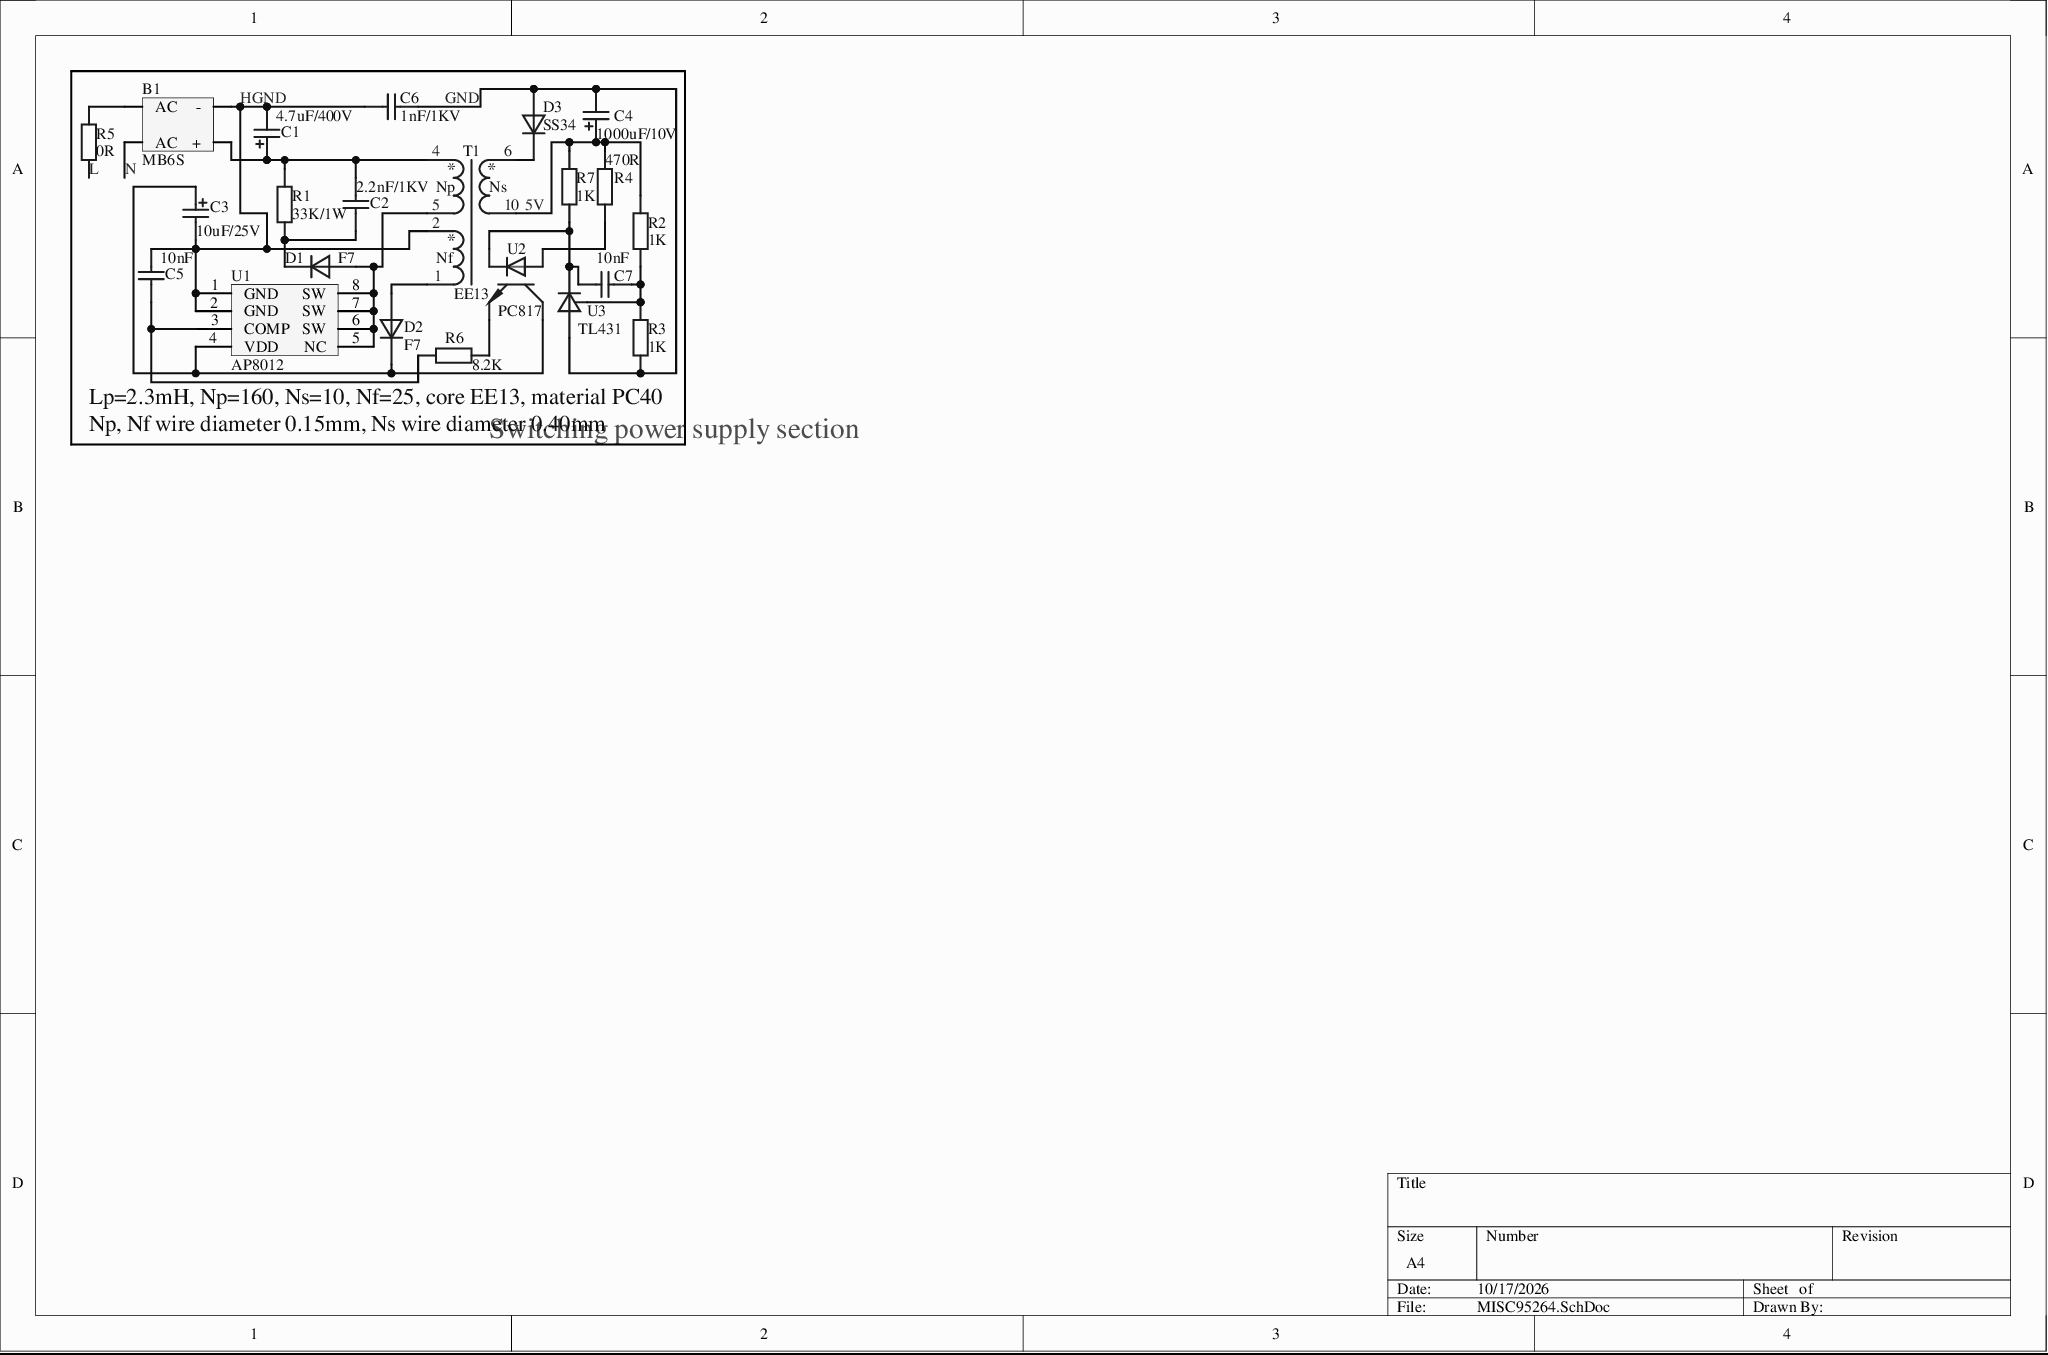
[diagram p0: MISC95264.SchDoc]
# Altium project MISC95264.PrjPcb
1 sheet, 22 parts. Net scope: global (net labels, ports and power ports of the same name join across sheets).
Board file: MISC95264.PcbDoc

## Sheet MISC95264.SchDoc
size A4

### Parts
B1  MB6S  [SOP4]
C1  4.7uF/400V  [cap-8*14mm]
C2  2.2nF/1KV  [CAP_5mm]
C3  10uF/25V  [cap-5*12mm]
C4  1000uF/10V  [cap-8*14mm]
C5  10nF  [0805_Cap]
C6  1nF/1KV  [CAP_5mm]
C7  10nF  [0805_Cap]
D1  F7  [SOD-123]
D2  F7  [SOD-123]
D3  SS34  [DO_214AC/SMA]
R1  33K/1W  [1W_Res_L]
R2  1K  [0805_Res]
R3  1K  [0805_Res]
R4  470R  [0805_Res]
R5  0R  [0805_Res]
R6  8.2K  [0805_Res]
R7  1K  [0805_Res]
T1  EE13  [EE13_5+5_L]
U1  AP8012  [DIP-8]
U2  PC817  [SOP4-PC817]
U3  TL431  [TO-92]

### Nets
5V: C4.1 R2.2 R4.2 R7.2 T1.10
GND: C4.2 C6.1 D3.1(A) R3.1 U3.2
HGND: B1.4(-) C1.2 C3.2 C5.2 C6.2 T1.2 U1.1(GND) U1.2(GND)
L: R5.1
N: B1.2(AC)
NetB1_1: B1.1(AC) R5.2
NetB1_3: B1.3(+) C1.1 C2.2 R1.1 T1.4
NetC2_1: C2.1 D1.2(K) R1.2
NetC3_1: C3.1 D2.2(K) U1.4(VDD) U2.4
NetC5_1: C5.1 R6.1 U1.3(COMP)
NetC7_1: C7.1 R7.1 U2.2 U3.3
NetC7_2: C7.2 R2.1 R3.2 U3.1
NetD1_1: D1.1(A) T1.5 U1.5(NC) U1.6(SW) U1.7(SW) U1.8(SW)
NetD2_1: D2.1(A) T1.1
NetD3_2: D3.2(K) T1.6
NetR4_1: R4.1 U2.1
NetR6_2: R6.2 U2.3

### Notes on the sheet
- (near T1) Np
- (near T1) Ns
- (near T1) Nf
- Lp=2.3mH, Np=160, Ns=10, Nf=25, core EE13, material PC40
- Np, Nf wire diameter 0.15mm, Ns wire diameter 0.40mm
- Switching power supply section

### Library data of the parts
B1 = MB6S: 600V 0.8A Bridge Rectifiers
C1 C3 C4 = Cap Pol
C2 C5-C7 = Cap
D1-D3 = Diode
R1-R7 = Res
T1 = Flyback transformer-1
U1 = AP8012: 5W Flyback SMPS Controller
U2 = PC817: Device Specification For PhotoCoupler
U3 = TL431: Adjustable Precision Shunt Regulator